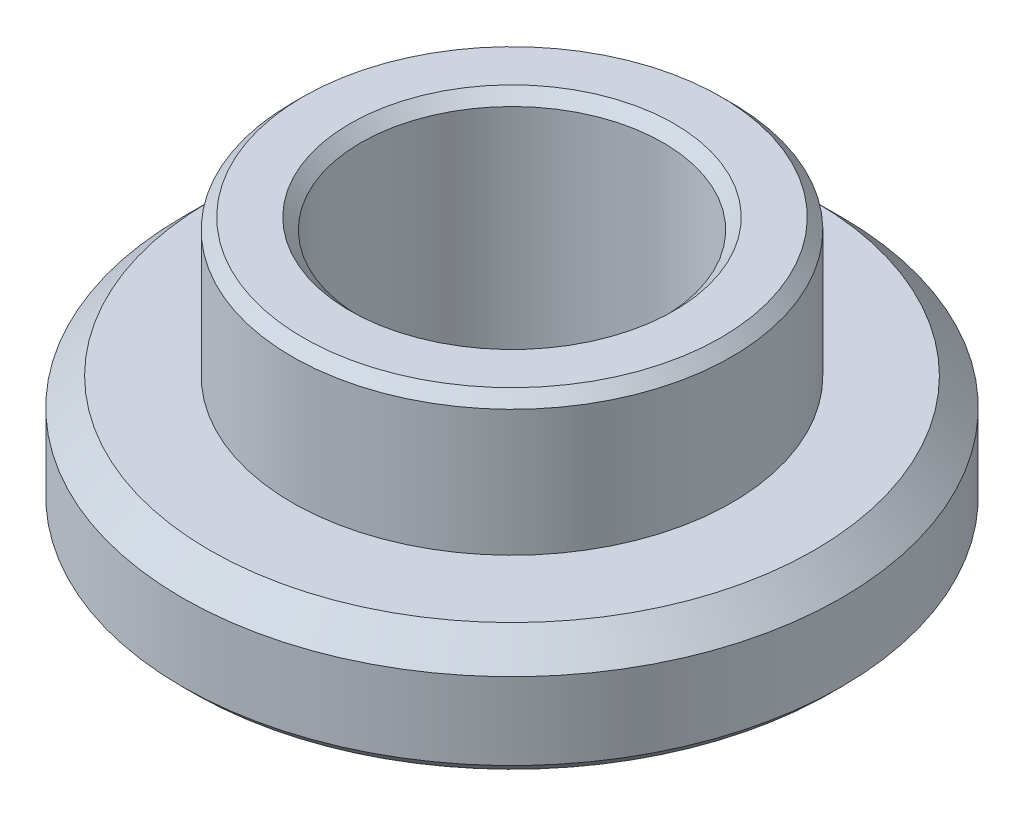
SolidWorks part; units mm, degrees
ref_plane "Front Plane" through (0, 0, 0) normal (0, 0, 1) x (1, 0, 0)
ref_plane "Top Plane" through (0, 0, 0) normal (0, 1, 0) x (1, 0, 0)
ref_plane "Right Plane" through (0, 0, 0) normal (1, 0, 0) x (0, 0, -1)
sketch "Sketch1" plane through (0, 0, 0) normal (0, 0, 1) x (1, 0, 0)
  line L0 (-29.5, 0) -> (-58, 0)
  line L1 (-60, 2) -> (-60, 16)
  line L2 (-55, 21) -> (-40, 21)
  line L3 (-40, 21) -> (-40, 44)
  line L4 (-38, 46) -> (-29.5, 46)
  line L5 (0, 46) -> (0, 0) construction
  line L6 (-27.5, 44) -> (-27.5, 2)
  line L7 (-58, 0) -> (-60, 2)
  line L8 (-27.5, 2) -> (-29.5, 0)
  line L9 (-29.5, 46) -> (-27.5, 44)
  line L12 (-60, 16) -> (-55, 21)
  line L13 (-40, 44) -> (-38, 46)
  point P1 (-60, 0)
  point P3 (-27.5, 0)
  point P4 (-60, 21)
  point P6 (-40, 46)
  point P9 (-27.5, 46)
  point P21 (-60, 21)
  point P24 (-40, 46)
  dimension "D1" = 60
  dimension "D2" = 21
  dimension "D3" = 25
  dimension "D4" = 40
  dimension "D5" = 27.5
revolve "Revolve1" add sketch "Sketch1" angle 360 about L5
